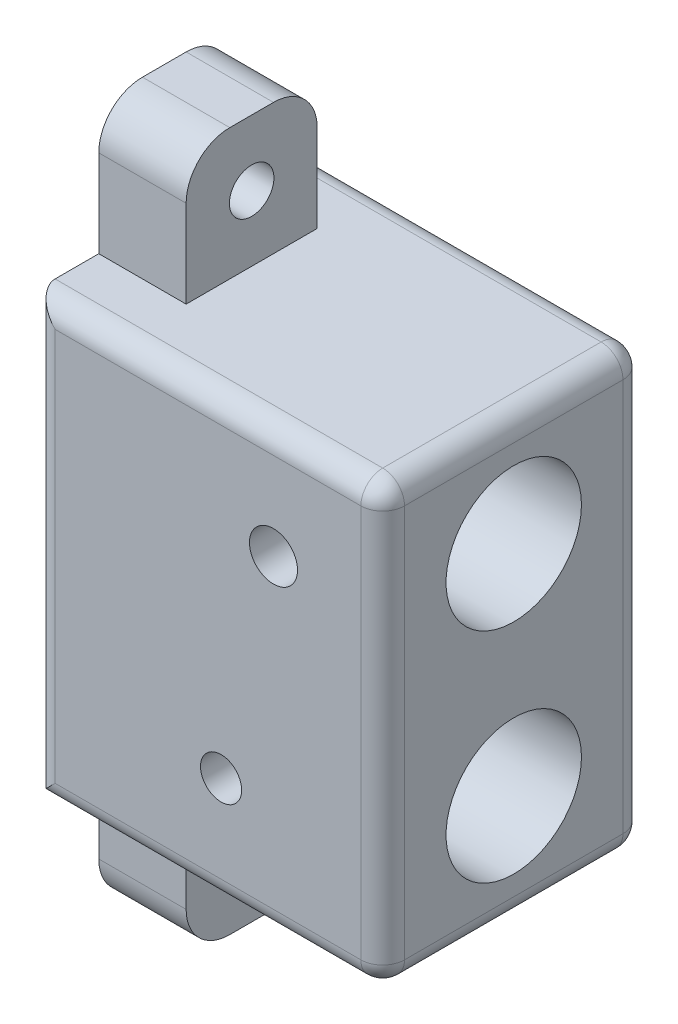
from build123d import *

# Parameters (mm, degrees)
BOSS_EXTRUDE1_DEPTH = 100
SKETCH2_R           = 15.5
CUT_EXTRUDE1_DEPTH  = 70
SKETCH3_R           = 5.1
CUT_EXTRUDE2_DEPTH  = 70
SKETCH4_R           = 5.5
SKETCH4_R_2         = 4.705316684
CUT_EXTRUDE3_DEPTH  = 70
SKETCH5_R           = 5.1
BOSS_EXTRUDE2_DEPTH = 20
SKETCH6_W           = 20
SKETCH6_H           = 100
CUT_EXTRUDE4_DEPTH  = 20
FILLET1_R           = 5


with BuildPart() as part:
    # Sketch1 → Boss-Extrude1 (new body)
    with BuildSketch(Plane(origin=(0, 0, 0), x_dir=(1, 0, 0), z_dir=(0, 1, 0))):
        Polygon((0, 20), (20, 20), (20, 0), (80, 0), (80, -60), (0, -60), (0, 0), align=None)
    extrude(amount=BOSS_EXTRUDE1_DEPTH)

    # Sketch2 → Cut-Extrude1 (cut)
    with BuildSketch(Plane(origin=(80, 0, 0), x_dir=(0, 0, -1), z_dir=(1, 0, 0))):
        with Locations((-30, 75)):
            Circle(SKETCH2_R)
        with Locations((-30, 25)):
            Circle(SKETCH2_R)
    extrude(amount=-CUT_EXTRUDE1_DEPTH, mode=Mode.SUBTRACT)

    # Sketch3 → Cut-Extrude2 (cut)
    with BuildSketch(Plane(origin=(20, 0, 0), x_dir=(0, 0, -1), z_dir=(1, 0, 0))):
        with Locations((10, 87.5)):
            Circle(SKETCH3_R)
        with Locations((10, 12.5)):
            Circle(SKETCH3_R)
        with Locations((10, 50)):
            Circle(SKETCH3_R)
    extrude(amount=-CUT_EXTRUDE2_DEPTH, mode=Mode.SUBTRACT)

    # Sketch4 → Cut-Extrude3 (cut)
    with BuildSketch(Plane(origin=(0, 0, 0), x_dir=(-1, 0, 0), z_dir=(0, 0, -1))):
        with Locations((-55, 75)):
            Circle(SKETCH4_R)
        with Locations((-43, 25)):
            Circle(SKETCH4_R_2)
    extrude(amount=-CUT_EXTRUDE3_DEPTH, mode=Mode.SUBTRACT)

    # Sketch5 → Boss-Extrude2 (add)
    with BuildSketch(Plane.ZY):
        with BuildLine():
            Line((25, 130), (35, 130))
            ThreePointArc((35, 130), (42.071067812, 127.071067812), (45, 120))
            Line((45, 120), (45, -20))
            ThreePointArc((45, -20), (42.071067812, -27.071067812), (35, -30))
            Line((35, -30), (25, -30))
            ThreePointArc((25, -30), (17.928932188, -27.071067812), (15, -20))
            Line((15, -20), (15, 120))
            ThreePointArc((15, 120), (17.928932188, 127.071067812), (25, 130))
        make_face()
        with Locations((30, 115)):
            Circle(SKETCH5_R, mode=Mode.SUBTRACT)
        with Locations((30, -15)):
            Circle(SKETCH5_R, mode=Mode.SUBTRACT)
    extrude(amount=-BOSS_EXTRUDE2_DEPTH)

    # Sketch6 → Cut-Extrude4 (cut)
    with BuildSketch(Plane(origin=(20, 0, 0), x_dir=(0, 0, -1), z_dir=(1, 0, 0))):
        with Locations((10, 50)):
            Rectangle(SKETCH6_W, SKETCH6_H)
    extrude(amount=-CUT_EXTRUDE4_DEPTH, mode=Mode.SUBTRACT)

    # Fillet1
    fillet1_edges = [part.edges().sort_by_distance(p)[0] for p in [
        (80, 100, 30),
        (80, 50, 0),
        (80, 50, 60),
        (0, 50, 60),
        (40, 100, 0),
        (0, 50, 0),
        (40, 100, 60),
        (40, 0, 0),
        (80, 0, 30),
        (40, 0, 60),
    ]]
    fillet(fillet1_edges, radius=FILLET1_R)


solid = part.part
